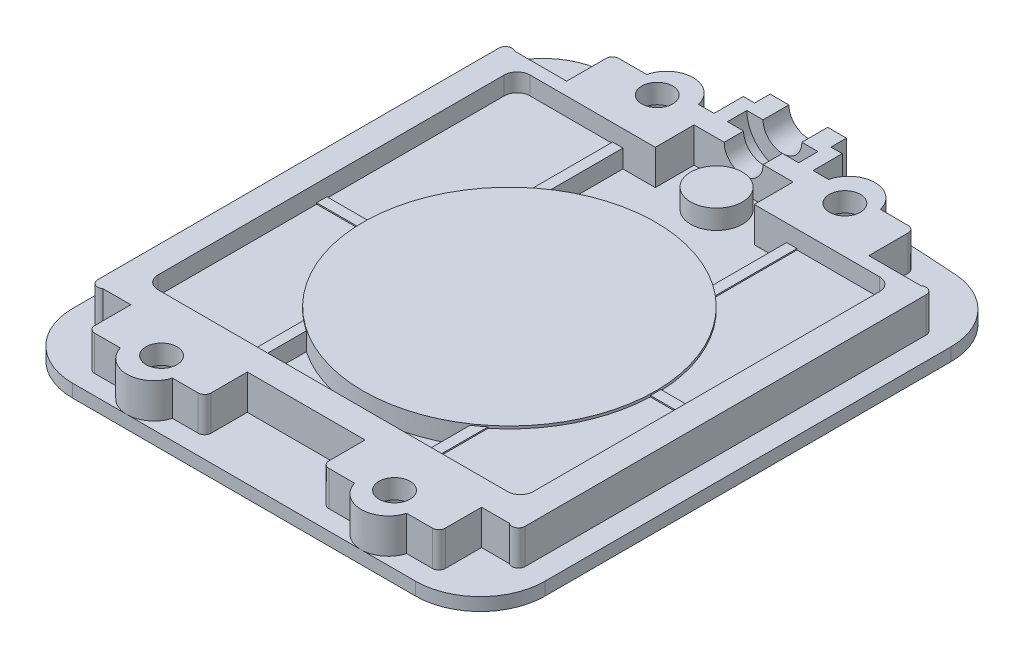
SolidWorks part; units mm, degrees
material "ABS"
ref_plane "Front Plane" through (0, 0, 0) normal (0, 0, 1) x (1, 0, 0)
ref_plane "Top Plane" through (0, 0, 0) normal (0, 1, 0) x (1, 0, 0)
ref_plane "Right Plane" through (0, 0, 0) normal (1, 0, 0) x (0, 0, -1)
sketch "Sketch 1" plane through (0, 0, 0) normal (0, 1, 0) x (1, 0, 0)
  line L0 (-18.25, 20.5) -> (18.25, -20.5) construction
  line L1 (-13.25, -20.5) -> (13.25, -20.5)
  line L2 (-18.25, -15.5) -> (-18.25, 15.8907)
  line L3 (-18.25, -20.5) -> (18.25, 20.5) construction
  line L4 (18.25, -15.5) -> (18.25, 15.8907)
  line L5 (0, 21.35) -> (0, -20.5) construction
  arc A0 (-13.5962, 20.8787) -> (13.5962, 20.8787) centre (0, -174.9941) cw
  arc A1 (18.25, 15.8907) -> (13.5962, 20.8787) centre (13.25, 15.8907) ccw
  arc A2 (-18.25, 15.8907) -> (-13.5962, 20.8787) centre (-13.25, 15.8907) cw
  arc A3 (13.25, -20.5) -> (18.25, -15.5) centre (13.25, -15.5) ccw
  arc A4 (-13.25, -20.5) -> (-18.25, -15.5) centre (-13.25, -15.5) cw
  point P0 (0, 0)
  point P1 (0, 0)
  dimension "D2" = 41
  dimension "D3" = 41.85
  dimension "D4" = 5
  dimension "D1" = 36.5
extrude "Boss-Extrude1" add sketch "Sketch 1" along normal blind 1
sketch "Sketch 2" plane through (0, 1, 0) normal (0, 1, 0) x (1, 0, 0)
  line L0 (0, 29.4306) -> (0, -25.9925) construction
  line L1 (-13.25, -20.5) -> (13.25, -20.5) construction
  line L2 (-13.55, -15.7022) -> (-15.7058, -15.7022)
  line L3 (-16.5058, -15.3022) -> (-16.5058, 15.6978)
  line L4 (-15.7058, 16.0978) -> (-11.675, 16.0978)
  line L5 (16.5058, -15.3022) -> (16.5058, 15.6978)
  line L6 (-16.5058, -15.3022) -> (16.7442, 16.0978) construction
  line L7 (-16.5058, 16.0451) -> (16.7442, -15.7022) construction
  line L8 (-3.825, 21.8978) -> (-3.825, 19.6378)
  line L9 (-4.55, -15.7022) -> (-4.55, -18.5)
  line L10 (-5.05, -19) -> (-7.0375, -19)
  line L11 (-13.55, -18.5) -> (-13.55, -15.7022)
  line L12 (-11.0625, -19) -> (-13.05, -19)
  line L13 (11.0625, -19) -> (13.05, -19)
  line L14 (13.55, -18.5) -> (13.55, -15.7022)
  line L15 (5.05, -19) -> (7.0375, -19)
  line L16 (4.55, -15.7022) -> (4.55, -18.5)
  line L17 (-4.55, -15.7022) -> (4.55, -15.7022)
  line L18 (13.55, -15.7022) -> (15.7058, -15.7022)
  line L19 (-16.625, 0.1978) -> (16.7442, 0.1978) construction
  line L20 (-9.025, 19.6378) -> (-11.175, 19.6378)
  line L21 (-11.675, 19.1378) -> (-11.675, 16.0978)
  line L22 (-3.825, 19.6378) -> (-5.025, 19.6378)
  line L23 (-14.5, -12.65) -> (-14.5, 14.0978)
  line L24 (14.5, -12.65) -> (14.5, 14.0978)
  line L25 (3.825, 19.6378) -> (5.025, 19.6378)
  line L26 (11.675, 19.1378) -> (11.675, 16.0978)
  line L27 (9.025, 19.6378) -> (11.175, 19.6378)
  line L28 (3.825, 21.8978) -> (3.825, 19.6378)
  line L29 (-13.5, -13.65) -> (13.5, -13.65)
  line L30 (3.825, 15.0978) -> (13.5, 15.0978)
  line L31 (-13.5, 15.0978) -> (-3.825, 15.0978)
  line L32 (15.7058, 16.0978) -> (11.675, 16.0978)
  line L33 (-14.5, -15.3022) -> (-14.5, 16.0451) construction
  line L34 (-3.825, 18.0978) -> (3.825, 18.0978)
  line L35 (-2.95, 23.0978) -> (2.95, 23.0978)
  line L36 (-3.825, 18.0978) -> (-3.825, 15.0978)
  line L37 (3.825, 18.0978) -> (3.825, 15.0978)
  line L38 (-16.5058, -15.3022) -> (-16.5058, 16.0451) construction
  line L39 (-15.7058, 15.0978) -> (-11.675, 15.0978) construction
  line L40 (-2.95, 23.0978) -> (-2.95, 21.8978)
  line L41 (-2.95, 21.8978) -> (-3.825, 21.8978)
  line L42 (-3.825, 23.0978) -> (3.825, 23.0978) construction
  line L43 (2.95, 21.8978) -> (3.825, 21.8978)
  line L44 (2.95, 23.0978) -> (2.95, 21.8978)
  arc A0 (-11.0625, -19) -> (-7.0375, -19) centre (-9.05, -18.4) ccw
  arc A1 (11.0625, -19) -> (7.0375, -19) centre (9.05, -18.4) cw
  arc A2 (-9.025, 19.6378) -> (-5.025, 19.6378) centre (-7.025, 19.1687) cw
  arc A3 (9.025, 19.6378) -> (5.025, 19.6378) centre (7.025, 19.1687) ccw
  arc A4 (-16.5058, 15.6978) -> (-15.7058, 16.0978) centre (-16.0058, 15.6978) cw
  arc A5 (-16.5058, -15.3022) -> (-15.7058, -15.7022) centre (-16.0058, -15.3022) ccw
  arc A6 (5.05, -19) -> (4.55, -18.5) centre (5.05, -18.5) cw
  arc A7 (16.5058, -15.3022) -> (15.7058, -15.7022) centre (16.0058, -15.3022) cw
  arc A8 (16.5058, 15.6978) -> (15.7058, 16.0978) centre (16.0058, 15.6978) ccw
  arc A9 (-13.5, -13.65) -> (-14.5, -12.65) centre (-13.5, -12.65) cw
  arc A10 (13.5, -13.65) -> (14.5, -12.65) centre (13.5, -12.65) ccw
  arc A11 (14.5, 14.0978) -> (13.5, 15.0978) centre (13.5, 14.0978) ccw
  arc A12 (-13.5, 15.0978) -> (-14.5, 14.0978) centre (-13.5, 14.0978) ccw
  arc A13 (13.05, -19) -> (13.55, -18.5) centre (13.05, -18.5) ccw
  arc A14 (-13.05, -19) -> (-13.55, -18.5) centre (-13.05, -18.5) cw
  arc A15 (11.675, 19.1378) -> (11.175, 19.6378) centre (11.175, 19.1378) ccw
  arc A16 (-11.175, 19.6378) -> (-11.675, 19.1378) centre (-11.175, 19.1378) ccw
  arc A17 (13.5962, 20.8787) -> (-13.5962, 20.8787) centre (0, -174.9941) ccw construction
  arc A18 (-4.55, -18.5) -> (-5.05, -19) centre (-5.05, -18.5) cw
  point P4 (0, 0.2853)
  point P74 (13.55, -19)
  point P77 (-13.55, -19)
  point P80 (11.675, 19.6378)
  point P83 (-11.675, 19.6378)
  point P89 (4.55, -19)
  point P92 (-4.55, -19)
  arc M3 (13.5962, 20.8787) -> (-13.5962, 20.8787) centre (0, -174.9941) ccw
  dimension "D5" = 2.1
  dimension "D8" = 3
  dimension "D11" = 5.9
  dimension "D17" = 0.5
  dimension "D3" = 32
  dimension "D18" = 0.5
  dimension "D19" = 0.5
  dimension "D2" = 1
  dimension "D10" = 8
  dimension "D4" = 9.1
  dimension "D6" = 9
  dimension "D7" = 1.5
  dimension "D9" = 23.35
  dimension "D12" = 31.8
  dimension "D13" = 4
  dimension "D14" = 7.65
  dimension "D15" = 29
  dimension "D16" = 1
  dimension "D20" = 1.2
  dimension "D21" = 1.2
extrude "Boss-Extrude3" add sketch "Sketch 2" along normal blind 2.7 and the other way blind 1 contours L20 A16 L21 L4 A4 L3 A5 L2 L11 A14 L12 A0 L10 L9 L17 L16 L15 A1 L13 A13 L14 L18 A7 L5 A8 L32 L26 A15 L27 A3 L25 L28 L8 L22 A2 A12 L31 L36 L34 L37 L30 A11 L24 A10 L29 A9 M3 | L35 L8 L28 M3
sketch "Sketch 4" plane through (0, 1, 0) normal (0, 1, 0) x (1, 0, 0)
  line L0 (-6.325, 15.0978) -> (-6.325, -13.65)
  line L1 (-13.5, 15.0978) -> (-3.825, 15.0978) construction
  line L2 (-13.5, -13.65) -> (13.5, -13.65) construction
  line L3 (-14.5, -12.65) -> (-14.5, 14.0978) construction
  line L4 (-13.5, -13.65) -> (13.5, -13.65) construction
  line L5 (-13.5, 15.0978) -> (-6.325, 15.0978)
  line L6 (-14.5, -12.65) -> (-14.5, 14.0978)
  line L7 (-13.5, -13.65) -> (-6.325, -13.65)
  line L8 (0, 26.1356) -> (0, -24.1425) construction
  line L9 (13.5, -13.65) -> (6.325, -13.65)
  line L10 (14.5, -12.65) -> (14.5, 14.0978)
  line L11 (13.5, 15.0978) -> (6.325, 15.0978)
  line L12 (6.325, 15.0978) -> (6.325, -13.65)
  arc A0 (-13.5, 15.0978) -> (-14.5, 14.0978) centre (-13.5, 14.0978) ccw construction
  arc A1 (-14.5, -12.65) -> (-13.5, -13.65) centre (-13.5, -12.65) ccw construction
  arc A2 (-13.5, 15.0978) -> (-14.5, 14.0978) centre (-13.5, 14.0978) ccw
  arc A3 (-14.5, -12.65) -> (-13.5, -13.65) centre (-13.5, -12.65) ccw
  arc A4 (14.5, -12.65) -> (13.5, -13.65) centre (13.5, -12.65) cw
  arc A5 (13.5, 15.0978) -> (14.5, 14.0978) centre (13.5, 14.0978) cw
  dimension "D1" = 2.5
extrude "Boss-Extrude4" add sketch "Sketch 4" along normal blind 1.3
sketch "Sketch 5" plane through (0, 2.3, 0) normal (0, 1, 0) x (1, 0, 0)
  line L0 (-6.325, 15.0978) -> (-6.325, -13.65)
  line L1 (-6.325, 15.0978) -> (-7.125, 15.0978)
  line L2 (-6.325, -13.65) -> (-7.125, -13.65)
  line L3 (-7.125, 15.0978) -> (-7.125, 0.4)
  line L4 (0, 18.0978) -> (0, -13.65) construction
  line L5 (-7.125, 0.4) -> (-14.5, 0.4)
  line L6 (-7.125, -0.4) -> (-14.5, -0.4)
  line L7 (-14.5, 0.4) -> (-14.5, -0.4)
  line L8 (-14.5, 14.0978) -> (-14.5, -12.65) construction
  line L9 (-7.125, -0.4) -> (-7.125, -13.65)
  line L10 (-3.825, 18.0978) -> (3.825, 18.0978) construction
  line L11 (-6.325, -13.65) -> (6.325, -13.65) construction
  line L12 (7.125, -0.4) -> (7.125, -13.65)
  line L13 (14.5, 0.4) -> (14.5, -0.4)
  line L14 (7.125, -0.4) -> (14.5, -0.4)
  line L15 (7.125, 0.4) -> (14.5, 0.4)
  line L16 (7.125, 15.0978) -> (7.125, 0.4)
  line L17 (6.325, -13.65) -> (7.125, -13.65)
  line L18 (6.325, 15.0978) -> (7.125, 15.0978)
  line L19 (6.325, 15.0978) -> (6.325, -13.65)
  point P6 (-14.5, 0)
  dimension "D1" = 0.8
  dimension "D2" = 0.8
extrude "Boss-Extrude5" add sketch "Sketch 5" along normal blind 0.1
sketch "Sketch 6" plane through (0, 1, 0) normal (0, 1, 0) x (1, 0, 0)
  circle A0 centre (0, 0) radius 11.3
  dimension "D1" = 22.6
extrude "Boss-Extrude6" add sketch "Sketch 6" along normal blind 1.5
sketch "Sketch 7" plane through (0, 0, 0) normal (1, 0, 0) x (0, 0, -1)
  line L0 (14.7388, 3.7) -> (24.4184, 3.7) construction
  line L1 (21.8978, 3.7) -> (19.6378, 3.7) construction
  line L2 (23.0978, 3.7) -> (23.0978, 2.2)
  line L3 (23.0978, 3.7) -> (18.0978, 3.7)
  line L4 (23.0978, 2.2) -> (21.0978, 2.2)
  line L5 (18.0978, 3.7) -> (18.0978, 2.2)
  line L6 (23.0978, 0) -> (23.0978, 3.7) construction
  line L7 (21.0978, 2.2) -> (21.0978, 0.95)
  line L9 (21.0978, 0.95) -> (19.5978, 0.95)
  line L10 (19.5978, 2.2) -> (19.5978, 0.95)
  line L11 (19.5978, 2.2) -> (18.0978, 2.2)
  dimension "D1" = 5
  dimension "D2" = 3
  dimension "D3" = 2
  dimension "D4" = 1.5
  dimension "D5" = 5.5
revolve "Cut-Revolve1" cut sketch "Sketch 7" angle 360 about L0
sketch "Sketch 8" plane through (0, 3.7, 0) normal (0, 1, 0) x (1, 0, 0)
  line L0 (0, 0) -> (0, 31.2249) construction
  circle A0 centre (-7.25, 18.673) radius 1.2
  circle A1 centre (9.05, -17.927) radius 1.2
  circle A2 centre (-8.9537, -17.927) radius 1.2
  circle A3 centre (9.05, -17.927) radius 1.2
  circle A4 centre (7.25, 18.673) radius 1.2
  arc A16 (-5.025, 19.6378) -> (-9.025, 19.6378) centre (-7.025, 19.1687) ccw construction
  point P33 (-7.025, 21.223)
  dimension "D1" = 1.2
  dimension "D2" = 14.5
  dimension "D3" = 36.6
  dimension "D4" = 1.35
extrude "Cut-Extrude1" cut sketch "Sketch 8" against normal up to surface (3.7 mm away) contours A1 | A2 | A0 | A4 up to face at (0, 0, -11.1147)
sketch "Sketch 9" plane through (0, 0, 0) normal (0, -1, 0) x (1, 0, 0)
  circle A0 centre (-8.9537, 17.927) radius 1.85
  circle A1 centre (9.05, 17.927) radius 1.85
  circle A2 centre (-7.25, -18.673) radius 1.85
  circle A3 centre (7.25, -18.673) radius 1.85
  circle A4 centre (0, 0) radius 9.175
  dimension "D1" = 1.85
  dimension "D2" = 9.175
extrude "Cut-Extrude2" cut sketch "Sketch 9" against normal blind 2.2
sketch "Sketch 10" plane through (0, 1, 0) normal (0, 1, 0) x (1, 0, 0)
  circle A0 centre (0, 16.009) radius 2
  dimension "D1" = 2
extrude "Boss-Extrude11" add sketch "Sketch 10" along normal blind 1.5
sketch "Sketch15" plane through (0, 1, 0) normal (0, 1, 0) x (1, 0, 0)
  line L0 (9.025, 19.6378) -> (11.175, 19.6378) construction
  line L1 (11.675, 19.1378) -> (11.675, 16.0978) construction
  line L2 (11.675, 16.0978) -> (15.7058, 16.0978) construction
  line L3 (16.5058, 15.6978) -> (16.5058, -15.3022) construction
  line L4 (15.7058, -15.7022) -> (13.55, -15.7022) construction
  line L5 (13.55, -15.7022) -> (13.55, -18.5) construction
  line L6 (13.05, -19) -> (11.0625, -19) construction
  line L7 (9.05, -20.5) -> (13.25, -20.5) construction
  line L8 (18.25, -15.5) -> (18.25, 15.8907) construction
  line L9 (-11.175, 19.6378) -> (-9.025, 19.6378)
  line L10 (-18.25, 15.8907) -> (-18.25, -15.5)
  line L11 (-13.25, -20.5) -> (-9.05, -20.5)
  line L12 (-11.0625, -19) -> (-13.05, -19)
  line L13 (-13.55, -18.5) -> (-13.55, -15.7022)
  line L14 (-13.55, -15.7022) -> (-15.7058, -15.7022)
  line L15 (-16.5058, -15.3022) -> (-16.5058, 15.6978)
  line L16 (-15.7058, 16.0978) -> (-11.675, 16.0978)
  line L17 (-11.675, 16.0978) -> (-11.675, 19.1378)
  line L18 (-11.175, 19.6378) -> (-9.025, 19.6378)
  line L19 (-18.25, 15.8907) -> (-18.25, -15.5)
  line L20 (-13.25, -20.5) -> (-9.05, -20.5)
  line L21 (-11.0625, -19) -> (-13.05, -19)
  line L22 (-13.55, -18.5) -> (-13.55, -15.7022)
  line L23 (-13.55, -15.7022) -> (-15.7058, -15.7022)
  line L24 (-16.5058, -15.3022) -> (-16.5058, 15.6978)
  line L25 (-15.7058, 16.0978) -> (-11.675, 16.0978)
  line L26 (-11.675, 16.0978) -> (-11.675, 19.1378)
  line L27 (-1.5, 19.5978) -> (-2.75, 19.5978) construction
  line L28 (-2.75, 21.0978) -> (-1.5, 21.0978) construction
  line L29 (-1.5, 23.0978) -> (-2.95, 23.0978) construction
  line L30 (-2.95, 23.0978) -> (-2.95, 21.8978) construction
  line L31 (-2.95, 21.8978) -> (-3.825, 21.8978) construction
  line L32 (-3.825, 21.8978) -> (-3.825, 19.6378) construction
  line L33 (-3.825, 19.6378) -> (-5.025, 19.6378) construction
  line L34 (-9.025, 19.6378) -> (-11.175, 19.6378) construction
  line L35 (-11.675, 19.1378) -> (-11.675, 16.0978) construction
  line L36 (-11.675, 16.0978) -> (-15.7058, 16.0978) construction
  line L37 (-16.5058, 15.6978) -> (-16.5058, -15.3022) construction
  line L38 (-15.7058, -15.7022) -> (-13.55, -15.7022) construction
  line L39 (-13.55, -15.7022) -> (-13.55, -18.5) construction
  line L40 (-13.05, -19) -> (-11.0625, -19) construction
  line L41 (-7.0375, -19) -> (-5.05, -19) construction
  line L42 (-4.55, -18.5) -> (-4.55, -15.7022) construction
  line L43 (-4.55, -15.7022) -> (4.55, -15.7022) construction
  line L44 (4.55, -15.7022) -> (4.55, -18.5) construction
  line L45 (5.05, -19) -> (7.0375, -19) construction
  line L46 (11.0625, -19) -> (13.05, -19) construction
  line L47 (13.55, -18.5) -> (13.55, -15.7022) construction
  line L48 (13.55, -15.7022) -> (15.7058, -15.7022) construction
  line L49 (16.5058, -15.3022) -> (16.5058, 15.6978) construction
  line L50 (15.7058, 16.0978) -> (11.675, 16.0978) construction
  line L51 (11.675, 16.0978) -> (11.675, 19.1378) construction
  line L52 (11.175, 19.6378) -> (9.025, 19.6378) construction
  line L53 (5.025, 19.6378) -> (3.825, 19.6378) construction
  line L54 (3.825, 19.6378) -> (3.825, 21.8978) construction
  line L55 (3.825, 21.8978) -> (2.95, 21.8978) construction
  line L56 (2.95, 21.8978) -> (2.95, 23.0978) construction
  line L57 (2.95, 23.0978) -> (1.5, 23.0978) construction
  line L58 (1.5, 21.0978) -> (2.75, 21.0978) construction
  line L59 (2.75, 19.5978) -> (1.5, 19.5978) construction
  line L60 (1.5, 18.0978) -> (3.825, 18.0978) construction
  line L61 (3.825, 18.0978) -> (3.825, 15.0978) construction
  line L62 (3.825, 15.0978) -> (13.5, 15.0978) construction
  line L63 (14.5, 14.0978) -> (14.5, -12.65) construction
  line L64 (13.5, -13.65) -> (-13.5, -13.65) construction
  line L65 (-14.5, -12.65) -> (-14.5, 14.0978) construction
  line L66 (-13.5, 15.0978) -> (-3.825, 15.0978) construction
  line L67 (-3.825, 15.0978) -> (-3.825, 18.0978) construction
  line L68 (-3.825, 18.0978) -> (-1.5, 18.0978) construction
  line L69 (-1.5, 21.0978) -> (1.5, 21.0978) construction
  line L70 (1.5, 23.0978) -> (-1.5, 23.0978) construction
  line L71 (-1.5, 18.0978) -> (1.5, 18.0978) construction
  line L72 (1.5, 19.5978) -> (-1.5, 19.5978) construction
  line L73 (2.75, 19.5978) -> (-2.75, 19.5978) construction
  line L74 (-2.75, 21.0978) -> (2.75, 21.0978) construction
  line L75 (9.025, 19.6378) -> (11.175, 19.6378)
  line L76 (11.675, 19.1378) -> (11.675, 16.0978)
  line L77 (11.675, 16.0978) -> (15.7058, 16.0978)
  line L78 (16.5058, 15.6978) -> (16.5058, -15.3022)
  line L79 (15.7058, -15.7022) -> (13.55, -15.7022)
  line L80 (13.55, -15.7022) -> (13.55, -18.5)
  line L81 (13.05, -19) -> (11.0625, -19)
  line L82 (9.05, -20.5) -> (13.25, -20.5)
  line L83 (18.25, -15.5) -> (18.25, 15.8907)
  line L84 (-1.5, 19.5978) -> (-2.75, 19.5978)
  line L85 (-2.75, 21.0978) -> (-1.5, 21.0978)
  line L86 (-1.5, 23.0978) -> (-2.95, 23.0978)
  line L87 (-2.95, 23.0978) -> (-2.95, 21.8978)
  line L88 (-2.95, 21.8978) -> (-3.825, 21.8978)
  line L89 (-3.825, 21.8978) -> (-3.825, 19.6378)
  line L90 (-3.825, 19.6378) -> (-5.025, 19.6378)
  line L91 (-9.025, 19.6378) -> (-11.175, 19.6378)
  line L92 (-11.675, 19.1378) -> (-11.675, 16.0978)
  line L93 (-11.675, 16.0978) -> (-15.7058, 16.0978)
  line L94 (-16.5058, 15.6978) -> (-16.5058, -15.3022)
  line L95 (-15.7058, -15.7022) -> (-13.55, -15.7022)
  line L96 (-13.55, -15.7022) -> (-13.55, -18.5)
  line L97 (-13.05, -19) -> (-11.0625, -19)
  line L98 (-7.0375, -19) -> (-5.05, -19)
  line L99 (-4.55, -18.5) -> (-4.55, -15.7022)
  line L100 (-4.55, -15.7022) -> (4.55, -15.7022)
  line L101 (4.55, -15.7022) -> (4.55, -18.5)
  line L102 (5.05, -19) -> (7.0375, -19)
  line L103 (11.0625, -19) -> (13.05, -19)
  line L104 (13.55, -18.5) -> (13.55, -15.7022)
  line L105 (13.55, -15.7022) -> (15.7058, -15.7022)
  line L106 (16.5058, -15.3022) -> (16.5058, 15.6978)
  line L107 (15.7058, 16.0978) -> (11.675, 16.0978)
  line L108 (11.675, 16.0978) -> (11.675, 19.1378)
  line L109 (11.175, 19.6378) -> (9.025, 19.6378)
  line L110 (5.025, 19.6378) -> (3.825, 19.6378)
  line L111 (3.825, 19.6378) -> (3.825, 21.8978)
  line L112 (3.825, 21.8978) -> (2.95, 21.8978)
  line L113 (2.95, 21.8978) -> (2.95, 23.0978)
  line L114 (2.95, 23.0978) -> (1.5, 23.0978)
  line L115 (1.5, 21.0978) -> (2.75, 21.0978)
  line L116 (2.75, 19.5978) -> (1.5, 19.5978)
  line L117 (1.5, 18.0978) -> (3.825, 18.0978)
  line L118 (3.825, 18.0978) -> (3.825, 15.0978)
  line L119 (3.825, 15.0978) -> (13.5, 15.0978)
  line L120 (14.5, 14.0978) -> (14.5, -12.65)
  line L121 (13.5, -13.65) -> (-13.5, -13.65)
  line L122 (-14.5, -12.65) -> (-14.5, 14.0978)
  line L123 (-13.5, 15.0978) -> (-3.825, 15.0978)
  line L124 (-3.825, 15.0978) -> (-3.825, 18.0978)
  line L125 (-3.825, 18.0978) -> (-1.5, 18.0978)
  line L126 (-1.5, 21.0978) -> (1.5, 21.0978)
  line L127 (1.5, 23.0978) -> (-1.5, 23.0978)
  line L128 (-1.5, 18.0978) -> (1.5, 18.0978)
  line L129 (1.5, 19.5978) -> (-1.5, 19.5978)
  line L130 (2.75, 19.5978) -> (-2.75, 19.5978)
  line L131 (-2.75, 21.0978) -> (2.75, 21.0978)
  arc A0 (9.025, 19.6378) -> (7.0993, 21.2216) centre (7.025, 19.1687) ccw construction
  arc A1 (11.675, 19.1378) -> (11.175, 19.6378) centre (11.175, 19.1378) ccw construction
  arc A2 (16.5058, 15.6978) -> (15.7058, 16.0978) centre (16.0058, 15.6978) ccw construction
  arc A3 (15.7058, -15.7022) -> (16.5058, -15.3022) centre (16.0058, -15.3022) ccw construction
  arc A4 (13.05, -19) -> (13.55, -18.5) centre (13.05, -18.5) ccw construction
  arc A5 (9.05, -20.5) -> (11.0625, -19) centre (9.05, -18.4) ccw construction
  arc A6 (13.25, -20.5) -> (18.25, -15.5) centre (13.25, -15.5) ccw construction
  arc A7 (18.25, 15.8907) -> (13.5962, 20.8787) centre (13.25, 15.8907) ccw construction
  arc A8 (13.5962, 20.8787) -> (7.0993, 21.2216) centre (0, -174.9941) ccw construction
  arc A9 (-7.0993, 21.2216) -> (-9.025, 19.6378) centre (-7.025, 19.1687) ccw
  arc A10 (-7.0993, 21.2216) -> (-13.5962, 20.8787) centre (0, -174.9941) ccw
  arc A11 (-13.5962, 20.8787) -> (-18.25, 15.8907) centre (-13.25, 15.8907) ccw
  arc A12 (-18.25, -15.5) -> (-13.25, -20.5) centre (-13.25, -15.5) ccw
  arc A13 (-11.0625, -19) -> (-9.05, -20.5) centre (-9.05, -18.4) ccw
  arc A14 (-13.55, -18.5) -> (-13.05, -19) centre (-13.05, -18.5) ccw
  arc A15 (-16.5058, -15.3022) -> (-15.7058, -15.7022) centre (-16.0058, -15.3022) ccw
  arc A16 (-15.7058, 16.0978) -> (-16.5058, 15.6978) centre (-16.0058, 15.6978) ccw
  arc A17 (-11.175, 19.6378) -> (-11.675, 19.1378) centre (-11.175, 19.1378) ccw
  arc A18 (-7.0993, 21.2216) -> (-9.025, 19.6378) centre (-7.025, 19.1687) ccw
  arc A19 (-7.0993, 21.2216) -> (-13.5962, 20.8787) centre (0, -174.9941) ccw
  arc A20 (-13.5962, 20.8787) -> (-18.25, 15.8907) centre (-13.25, 15.8907) ccw
  arc A21 (-18.25, -15.5) -> (-13.25, -20.5) centre (-13.25, -15.5) ccw
  arc A22 (-11.0625, -19) -> (-9.05, -20.5) centre (-9.05, -18.4) ccw
  arc A23 (-13.55, -18.5) -> (-13.05, -19) centre (-13.05, -18.5) ccw
  arc A24 (-16.5058, -15.3022) -> (-15.7058, -15.7022) centre (-16.0058, -15.3022) ccw
  arc A25 (-15.7058, 16.0978) -> (-16.5058, 15.6978) centre (-16.0058, 15.6978) ccw
  arc A26 (-11.175, 19.6378) -> (-11.675, 19.1378) centre (-11.175, 19.1378) ccw
  arc A27 (-5.025, 19.6378) -> (-9.025, 19.6378) centre (-7.025, 19.1687) ccw construction
  arc A28 (-11.175, 19.6378) -> (-11.675, 19.1378) centre (-11.175, 19.1378) ccw construction
  arc A29 (-15.7058, 16.0978) -> (-16.5058, 15.6978) centre (-16.0058, 15.6978) ccw construction
  arc A30 (-16.5058, -15.3022) -> (-15.7058, -15.7022) centre (-16.0058, -15.3022) ccw construction
  arc A31 (-13.55, -18.5) -> (-13.05, -19) centre (-13.05, -18.5) ccw construction
  arc A32 (-11.0625, -19) -> (-7.0375, -19) centre (-9.05, -18.4) ccw construction
  arc A33 (-5.05, -19) -> (-4.55, -18.5) centre (-5.05, -18.5) ccw construction
  arc A34 (4.55, -18.5) -> (5.05, -19) centre (5.05, -18.5) ccw construction
  arc A35 (7.0375, -19) -> (11.0625, -19) centre (9.05, -18.4) ccw construction
  arc A36 (13.05, -19) -> (13.55, -18.5) centre (13.05, -18.5) ccw construction
  arc A37 (15.7058, -15.7022) -> (16.5058, -15.3022) centre (16.0058, -15.3022) ccw construction
  arc A38 (16.5058, 15.6978) -> (15.7058, 16.0978) centre (16.0058, 15.6978) ccw construction
  arc A39 (11.675, 19.1378) -> (11.175, 19.6378) centre (11.175, 19.1378) ccw construction
  arc A40 (9.025, 19.6378) -> (5.025, 19.6378) centre (7.025, 19.1687) ccw construction
  arc A41 (14.5, 14.0978) -> (13.5, 15.0978) centre (13.5, 14.0978) ccw construction
  arc A42 (13.5, -13.65) -> (14.5, -12.65) centre (13.5, -12.65) ccw construction
  arc A43 (-14.5, -12.65) -> (-13.5, -13.65) centre (-13.5, -12.65) ccw construction
  arc A44 (-13.5, 15.0978) -> (-14.5, 14.0978) centre (-13.5, 14.0978) ccw construction
  circle A45 centre (0, 0) radius 11.3 construction
  arc A46 (9.025, 19.6378) -> (7.0993, 21.2216) centre (7.025, 19.1687) ccw
  arc A47 (11.675, 19.1378) -> (11.175, 19.6378) centre (11.175, 19.1378) ccw
  arc A48 (16.5058, 15.6978) -> (15.7058, 16.0978) centre (16.0058, 15.6978) ccw
  arc A49 (15.7058, -15.7022) -> (16.5058, -15.3022) centre (16.0058, -15.3022) ccw
  arc A50 (13.05, -19) -> (13.55, -18.5) centre (13.05, -18.5) ccw
  arc A51 (9.05, -20.5) -> (11.0625, -19) centre (9.05, -18.4) ccw
  arc A52 (13.25, -20.5) -> (18.25, -15.5) centre (13.25, -15.5) ccw
  arc A53 (18.25, 15.8907) -> (13.5962, 20.8787) centre (13.25, 15.8907) ccw
  arc A54 (13.5962, 20.8787) -> (7.0993, 21.2216) centre (0, -174.9941) ccw
  arc A55 (-5.025, 19.6378) -> (-9.025, 19.6378) centre (-7.025, 19.1687) ccw
  arc A56 (-11.175, 19.6378) -> (-11.675, 19.1378) centre (-11.175, 19.1378) ccw
  arc A57 (-15.7058, 16.0978) -> (-16.5058, 15.6978) centre (-16.0058, 15.6978) ccw
  arc A58 (-16.5058, -15.3022) -> (-15.7058, -15.7022) centre (-16.0058, -15.3022) ccw
  arc A59 (-13.55, -18.5) -> (-13.05, -19) centre (-13.05, -18.5) ccw
  arc A60 (-11.0625, -19) -> (-7.0375, -19) centre (-9.05, -18.4) ccw
  arc A61 (-5.05, -19) -> (-4.55, -18.5) centre (-5.05, -18.5) ccw
  arc A62 (4.55, -18.5) -> (5.05, -19) centre (5.05, -18.5) ccw
  arc A63 (7.0375, -19) -> (11.0625, -19) centre (9.05, -18.4) ccw
  arc A64 (13.05, -19) -> (13.55, -18.5) centre (13.05, -18.5) ccw
  arc A65 (15.7058, -15.7022) -> (16.5058, -15.3022) centre (16.0058, -15.3022) ccw
  arc A66 (16.5058, 15.6978) -> (15.7058, 16.0978) centre (16.0058, 15.6978) ccw
  arc A67 (11.675, 19.1378) -> (11.175, 19.6378) centre (11.175, 19.1378) ccw
  arc A68 (9.025, 19.6378) -> (5.025, 19.6378) centre (7.025, 19.1687) ccw
  arc A69 (14.5, 14.0978) -> (13.5, 15.0978) centre (13.5, 14.0978) ccw
  arc A70 (13.5, -13.65) -> (14.5, -12.65) centre (13.5, -12.65) ccw
  arc A71 (-14.5, -12.65) -> (-13.5, -13.65) centre (-13.5, -12.65) ccw
  arc A72 (-13.5, 15.0978) -> (-14.5, 14.0978) centre (-13.5, 14.0978) ccw
  circle A73 centre (0, 0) radius 11.3
  dimension "D1" = 0
